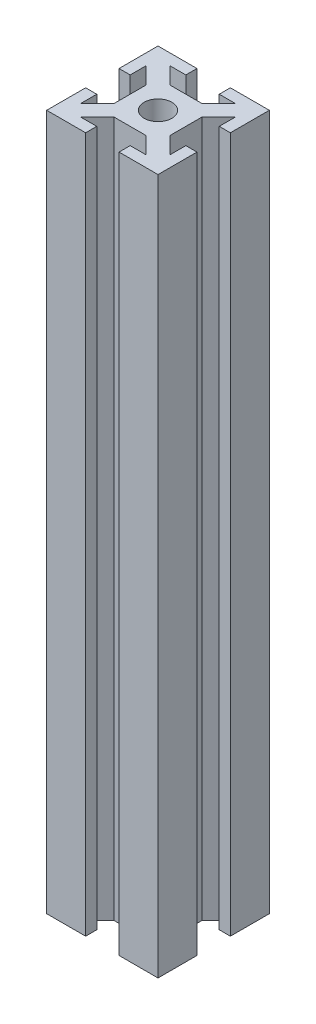
from build123d import *

# Parameters (mm, degrees)
SKETCH1_R           = 5
BOSS_EXTRUDE1_DEPTH = 250


with BuildPart() as part:
    # Sketch1 → Boss-Extrude1 (new body)
    with BuildSketch(Plane(origin=(0, 0, 0), x_dir=(1, 0, 0), z_dir=(0, 1, 0))):
        Polygon((-6, 20), (-6, 16), (-11.757359313, 16), (-5.757359313, 10), (5.757359313, 10), (11.757359313, 16), (6, 16), (6, 20), (20, 20), (20, 6), (16, 6), (16, 11.757359313), (10, 5.757359313), (10, -5.757359313), (16, -11.757359313), (16, -6), (20, -6), (20, -20), (6, -20), (6, -16), (11.757359313, -16), (5.757359313, -10), (-5.757359313, -10), (-11.757359313, -16), (-6, -16), (-6, -20), (-20, -20), (-20, -6), (-16, -6), (-16, -11.757359313), (-10, -5.757359313), (-10, 5.757359313), (-16, 11.757359313), (-16, 6), (-20, 6), (-20, 20), align=None)
        with Locations(Location((0, 0, 0), (0, 0, 270))):
            Circle(SKETCH1_R, mode=Mode.SUBTRACT)
    extrude(amount=BOSS_EXTRUDE1_DEPTH)


solid = part.part
